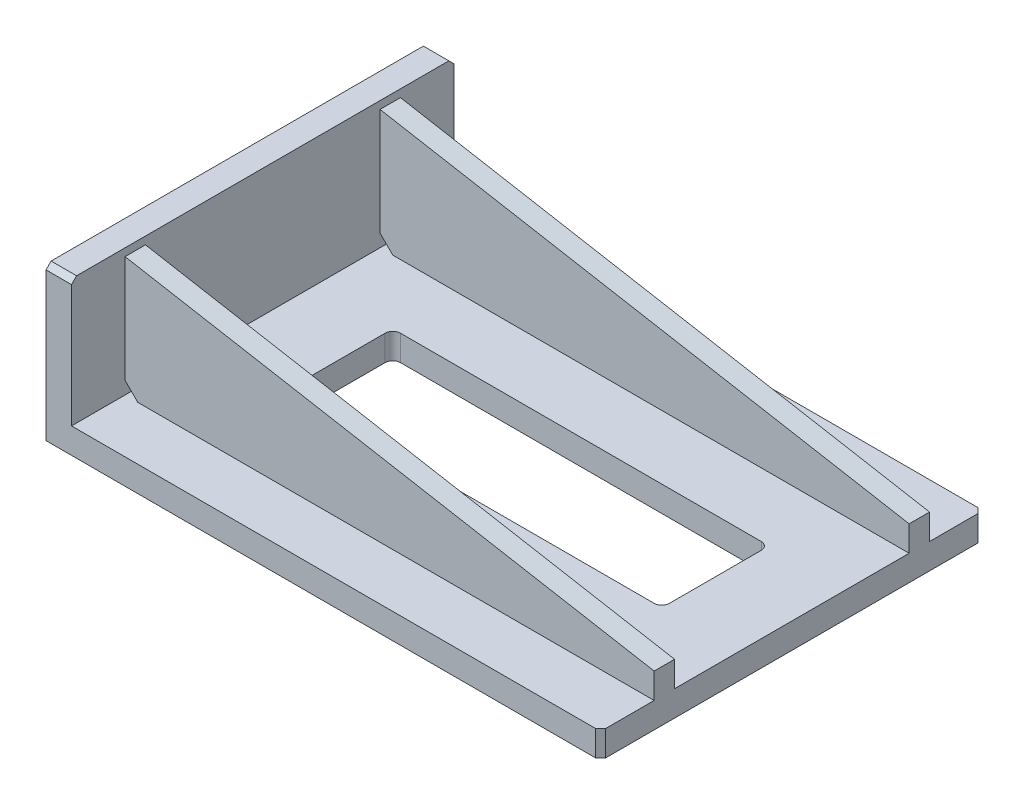
from build123d import *

# Parameters (mm, degrees)
EXTRUDE_1_DEPTH     = 75
EXTRUDE_START       = 50
EXTRUDE_2_DEPTH     = 4
CHAMFER_1_SIZE      = 2
CUT_EXTRUDE_1_REACH = 237.438
SKETCH_3_W          = 147.5
SKETCH_3_H          = 42
FILLET_1_R          = 3


with BuildPart() as part:
    # 草图1 → 凸台-拉伸1 (new, symmetric)
    with BuildSketch(Plane.XY):
        Polygon((0, 0), (217.5, 0), (217.5, 10), (10, 10), (10, 60), (0, 60), align=None)
    extrude(amount=EXTRUDE_1_DEPTH, both=True)

    # 草图2 → 凸台-拉伸2 (add, symmetric)
    with BuildSketch(Plane.XY.offset(EXTRUDE_START)):
        Polygon((10, 57), (217.5, 20), (217.5, 10), (15, 10), (10, 15), align=None)
    extrude_2 = extrude(amount=EXTRUDE_2_DEPTH, both=True)

    # 倒角1
    chamfer_1_edges = [part.edges().sort_by_distance(p)[0] for p in [
        (217.5, 5, 75),
        (5, 60, 75),
        (5, 60, -75),
        (217.5, 5, -75),
    ]]
    chamfer(chamfer_1_edges, length=CHAMFER_1_SIZE)

    # 镜向1: 凸台-拉伸2 across plane
    add(extrude_2.mirror(Plane.XY))

    # 草图3 → 切除-拉伸1 (cut, up to next)
    with BuildSketch(Plane(origin=(0, 10, 0), x_dir=(1, 0, 0), z_dir=(0, 1, 0)), mode=Mode.PRIVATE) as cut_extrude_1_sk1:
        with Locations((113.75, 0)):
            Rectangle(SKETCH_3_W, SKETCH_3_H)
    cut_extrude_1_tool1 = extrude(cut_extrude_1_sk1.sketch, amount=-CUT_EXTRUDE_1_REACH, mode=Mode.PRIVATE) & part.part
    add(cut_extrude_1_tool1.solids().sort_by_distance((113.75, 10, 0))[0], mode=Mode.SUBTRACT)

    # 圆角1
    fillet_1_edges = [part.edges().sort_by_distance(p)[0] for p in [
        (187.5, 5, -21),
        (187.5, 5, 21),
        (40, 5, 21),
        (40, 5, -21),
    ]]
    fillet(fillet_1_edges, radius=FILLET_1_R)


solid = part.part
